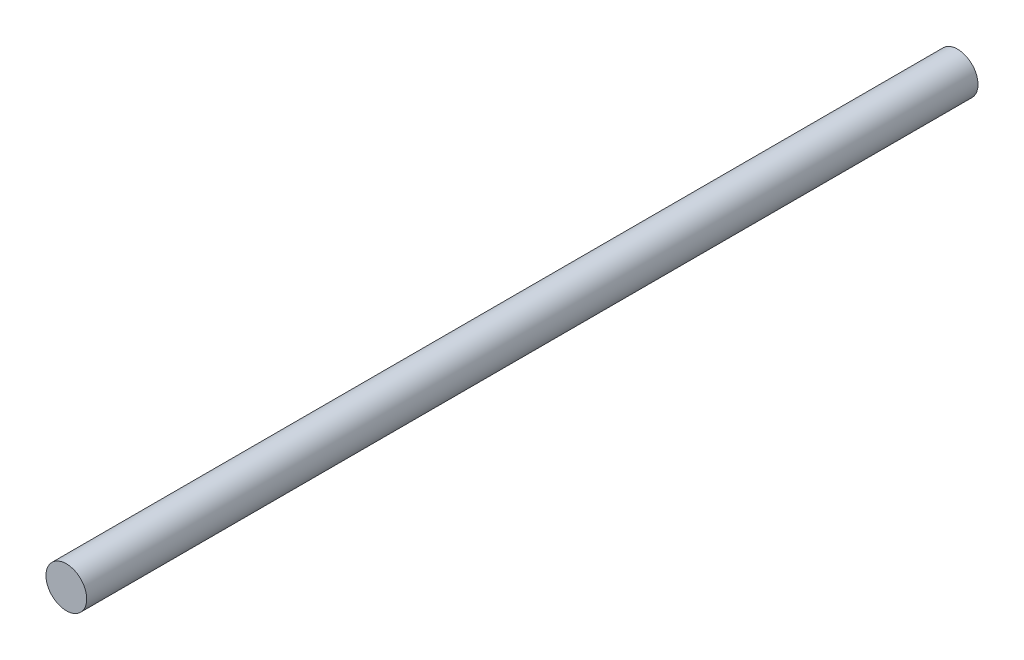
SolidWorks part; units mm, degrees
ref_plane "前视基准面" through (0, 0, 0) normal (0, 0, 1) x (1, 0, 0)
ref_plane "上视基准面" through (0, 0, 0) normal (0, 1, 0) x (1, 0, 0)
ref_plane "右视基准面" through (0, 0, 0) normal (1, 0, 0) x (0, 0, -1)
sketch "草图1" plane through (0, 0, 0) normal (0, 0, 1) x (1, 0, 0)
  circle A0 centre (0, 0) radius 8
  dimension "D1" = 16
extrude "凸台-拉伸1" add sketch "草图1" along normal blind 350
cosmetic thread "装饰螺纹线1" parameters "D1"=50, "D2"=15
cosmetic thread "装饰螺纹线2" parameters "D1"=50, "D2"=15
cosmetic thread "装饰螺纹线3" parameters "D1"=50, "D2"=15
